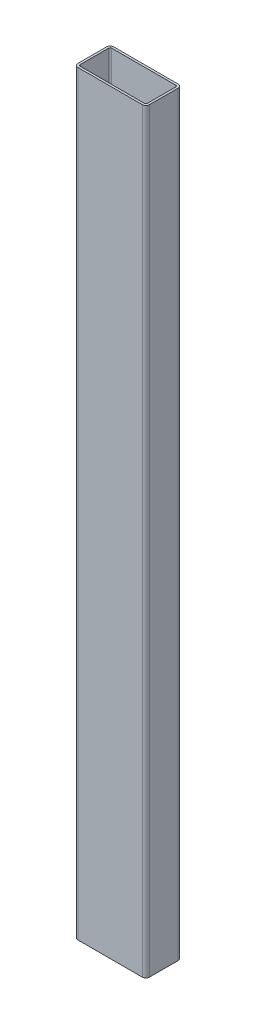
SolidWorks part; units mm, degrees
ref_plane "Front Plane" through (0, 0, 0) normal (0, 0, 1) x (1, 0, 0)
ref_plane "Top Plane" through (0, 0, 0) normal (0, 1, 0) x (1, 0, 0)
ref_plane "Right Plane" through (0, 0, 0) normal (1, 0, 0) x (0, 0, -1)
other "Configuration Table"
sketch "Sketch1" plane through (0, 0, 0) normal (0, 1, 0) x (1, 0, 0)
  line L1 (-90, 50) -> (90, 50)
  line L2 (-100, 40) -> (-100, -40)
  line L3 (-90, -50) -> (90, -50)
  line L4 (100, 40) -> (100, -40)
  line L5 (-100, 50) -> (100, -50) construction
  line L6 (-100, -50) -> (100, 50) construction
  arc A0 (90, 50) -> (100, 40) centre (90, 40) cw
  arc A1 (90, -50) -> (100, -40) centre (90, -40) ccw
  arc A2 (-100, -40) -> (-90, -50) centre (-90, -40) ccw
  arc A3 (-90, 50) -> (-100, 40) centre (-90, 40) ccw
  point P0 (0, 0)
  dimension "D3" = 10
  dimension "D1" = 200
  dimension "D2" = 100
extrude "Extrude-Thin1" add sketch "Sketch1" along normal mid plane 2114 thin
